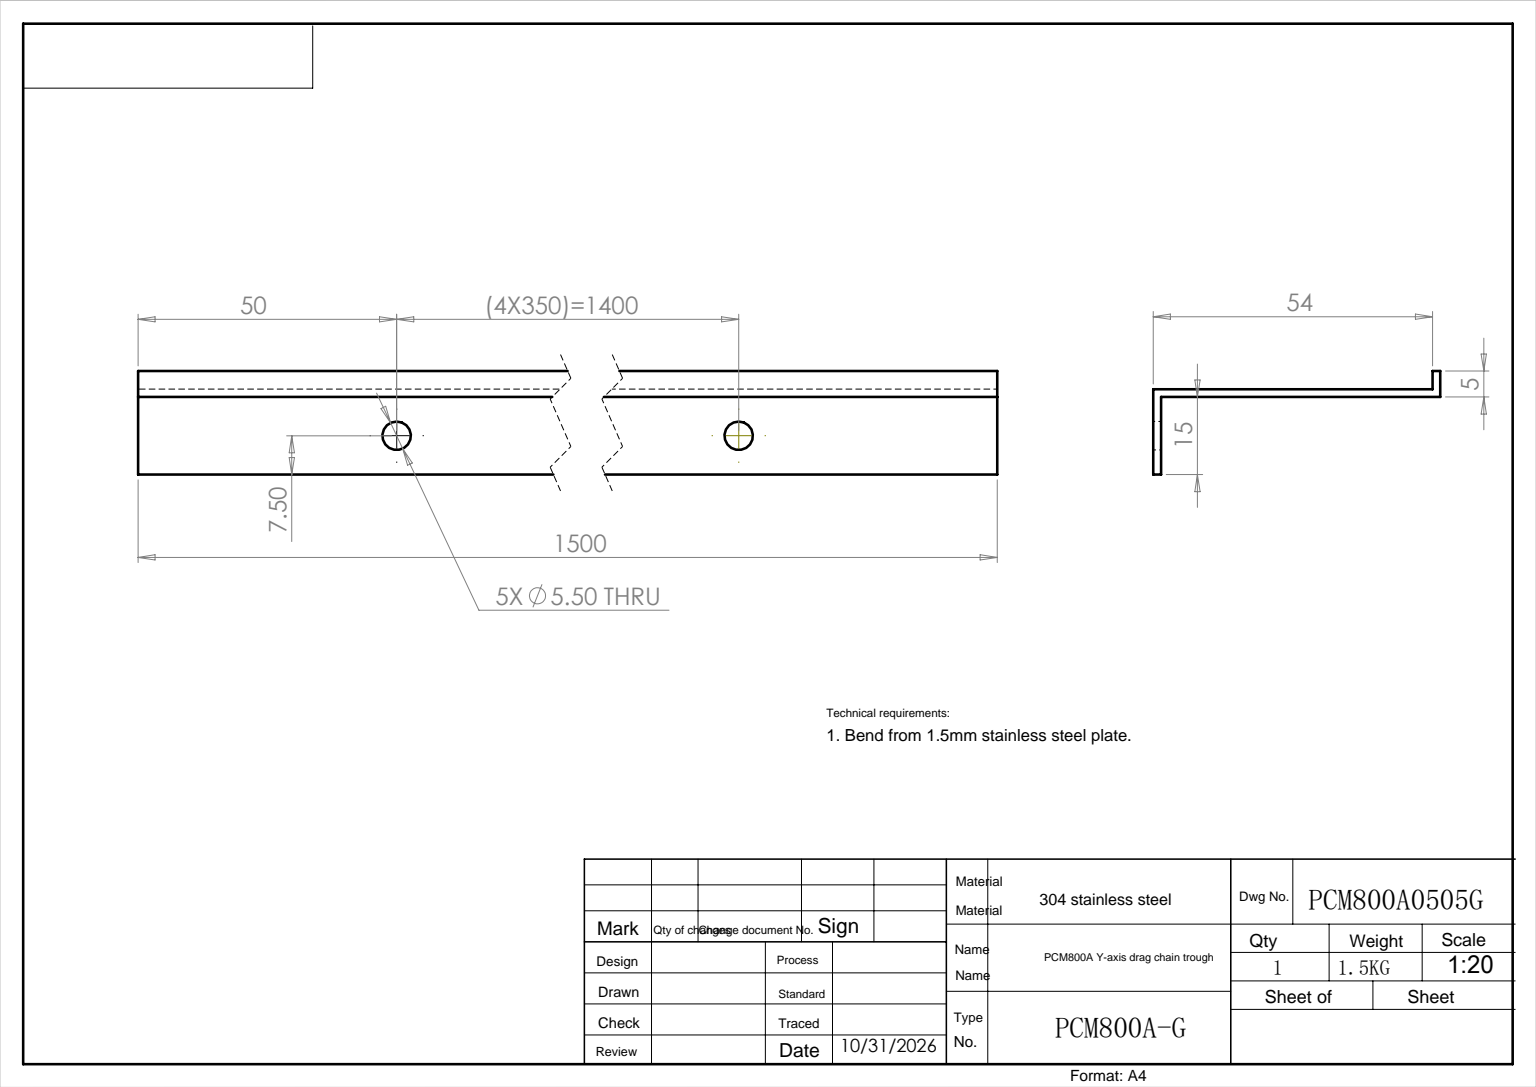
from build123d import *

# Parameters (mm, degrees)
EXTRUDE_1_DEPTH     = 1500
SKETCH_2_R          = 2.75
CUT_EXTRUDE_1_DEPTH = 10


with BuildPart() as part:
    # 草图1 → 拉伸-薄壁1 (new body)
    with BuildSketch(Plane.XY):
        Polygon((54, 5), (54, 0), (0, 0), (0, -15), (-1.5, -15), (-1.5, 1.5), (52.5, 1.5), (52.5, 5), align=None)
    extrude(amount=EXTRUDE_1_DEPTH)

    # 草图2 → 切除-拉伸1 (cut)
    with BuildSketch(Plane(origin=(0, 0, 0), x_dir=(0, 0, -1), z_dir=(1, 0, 0))):
        with Locations(Location((-1450, -7.5, 0), (0, 0, 90))):
            Circle(SKETCH_2_R)
        with Locations(Location((-1100, -7.5, 0), (0, 0, 90))):
            Circle(SKETCH_2_R)
        with Locations(Location((-750, -7.5, 0), (0, 0, 90))):
            Circle(SKETCH_2_R)
        with Locations(Location((-400, -7.5, 0), (0, 0, 90))):
            Circle(SKETCH_2_R)
        with Locations(Location((-50, -7.5, 0), (0, 0, 90))):
            Circle(SKETCH_2_R)
    extrude(amount=-CUT_EXTRUDE_1_DEPTH, mode=Mode.SUBTRACT)


solid = part.part
